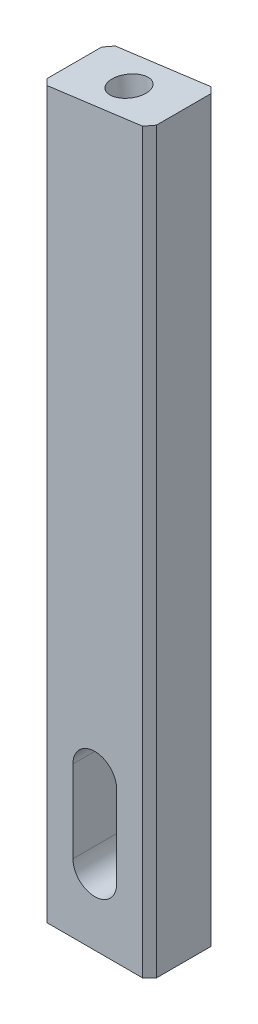
from build123d import *

# Parameters (mm, degrees)
SKETCH1_W             = 8
SKETCH1_H             = 54
BOSS_EXTRUDE1_DEPTH   = 2.5
CUT_EXTRUDE1_DEPTH    = 28.748873851
M3_TAPPED_HOLE1_D     = 2.5
M3_TAPPED_HOLE1_DEPTH = 8.5
M3_TAPPED_HOLE1_TIP   = 0.751075774
CUT_EXTRUDE2_DEPTH    = 28.748873851
CHAMFER1_SIZE         = 0.5


with BuildPart() as part:
    # Sketch1 → Boss-Extrude1 (new, symmetric)
    with BuildSketch(Plane.XY):
        Rectangle(SKETCH1_W, SKETCH1_H)
    extrude(amount=BOSS_EXTRUDE1_DEPTH, both=True)

    # Sketch2 → Cut-Extrude1 (cut, through all)
    with BuildSketch(Plane.XY.offset(2.5)):
        Polygon((4, 27), (-4, 27), (-4, 25.946780019), align=None)
    extrude(amount=-CUT_EXTRUDE1_DEPTH, mode=Mode.SUBTRACT)

    # M3 Tapped Hole1
    with Locations(Plane(origin=(-3.425908761, 26.022360565, 0), x_dir=(0.9914448613738103, 0.13052619222005266, 0), z_dir=(-0.13052619222005266, 0.9914448613738103, 0))):
        with Locations((3.455470793, 0)):
            Hole(M3_TAPPED_HOLE1_D / 2, depth=M3_TAPPED_HOLE1_DEPTH)
            with Locations((0, 0, -(M3_TAPPED_HOLE1_DEPTH + M3_TAPPED_HOLE1_TIP / 2))):  # 118° drill point
                Cone(0, M3_TAPPED_HOLE1_D / 2, M3_TAPPED_HOLE1_TIP, mode=Mode.SUBTRACT)

    # Sketch5 → Cut-Extrude2 (cut, through all)
    with BuildSketch(Plane.XY.offset(2.5)):
        with BuildLine():
            Line((-1.6, -22), (-1.6, -16))
            ThreePointArc((-1.6, -16), (0, -14.4), (1.6, -16))
            Line((1.6, -16), (1.6, -22))
            ThreePointArc((1.6, -22), (0, -23.6), (-1.6, -22))
        make_face()
    extrude(amount=-CUT_EXTRUDE2_DEPTH, mode=Mode.SUBTRACT)

    # Chamfer1
    chamfer1_edges = [part.edges().sort_by_distance(p)[0] for p in [
        (-4, -0.52660999, -2.5),
        (-4, -0.52660999, 2.5),
        (4, 0, 2.5),
        (4, 0, -2.5),
    ]]
    chamfer(chamfer1_edges, length=CHAMFER1_SIZE)


solid = part.part
